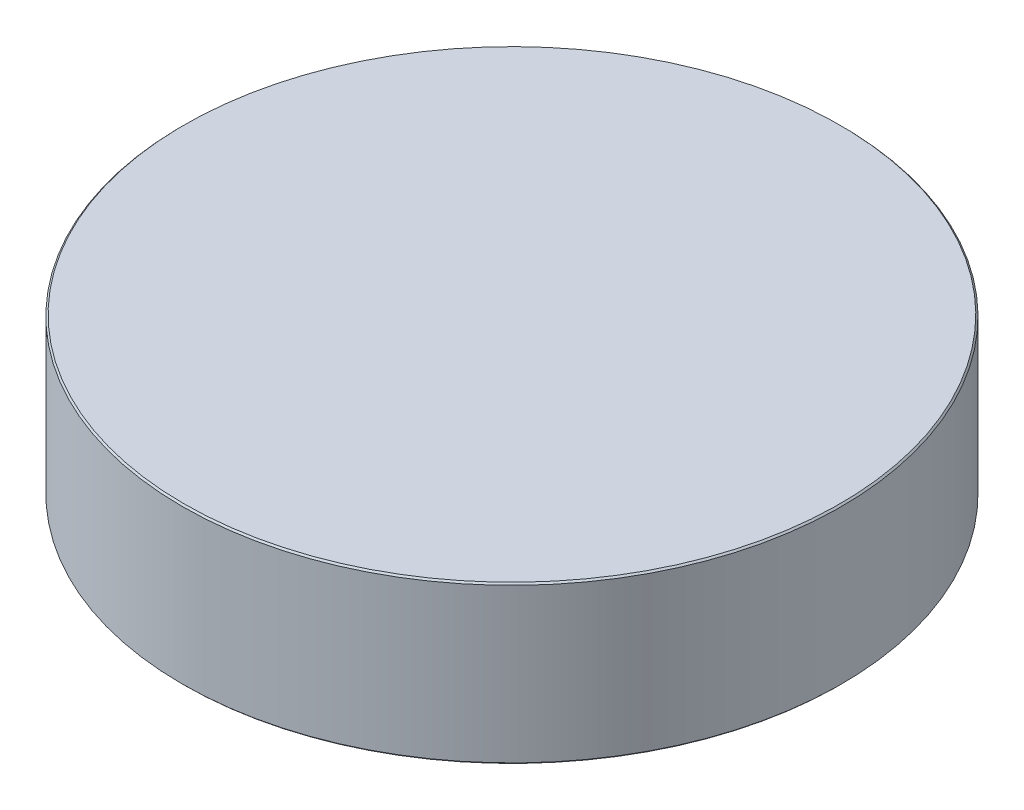
from build123d import *

# Parameters (mm, degrees)
SKETCH_1_R               = 210
SKETCH_1_R_2             = 95.82
EXTRUDE_1_DEPTH          = 100
SKETCH_5_R               = 150
EXTRUDE_4_DEPTH          = 30
PATTERN_CIRCULAR_1_COUNT = 8
CHAMFER_1_SIZE           = 1


with BuildPart() as part:
    # 草图1 → 凸台-拉伸1 (new body)
    with BuildSketch(Plane(origin=(0, 0, 0), x_dir=(1, 0, 0), z_dir=(0, 1, 0))):
        with Locations(Location((0, 0, 0), (0, 0, 270))):
            Circle(SKETCH_1_R)
        with Locations(Location((0, 0, 0), (0, 0, 270))):
            Circle(SKETCH_1_R_2, mode=Mode.SUBTRACT)
    extrude(amount=EXTRUDE_1_DEPTH)

    # 草图5 → 凸台-拉伸4 (add)
    with BuildSketch(Plane(origin=(0, 100, 0), x_dir=(1, 0, 0), z_dir=(0, 1, 0))):
        Circle(SKETCH_5_R)
    extrude(amount=-EXTRUDE_4_DEPTH)

    # 草图8 → M10 螺纹孔1 (revolve, cut)
    with BuildSketch(Plane(origin=(185, 0, 0), x_dir=(0, 0, -1), z_dir=(1, 0, 0))):
        Polygon((0, 0), (0, 30.053657631), (4.25, 27.5), (4.25, 0.775), (5.025, 0), align=None)
    hole_wizard_m10_1 = revolve(axis=Axis((185, -6.35, 0), (0, 1, 0)), mode=Mode.SUBTRACT)

    # 阵列(圆周)1: M10 螺纹孔1 ×8 about axis
    pattern_circular_1_axis = Axis((0, 0, 0), (0, 1, 0))
    for i in range(1, PATTERN_CIRCULAR_1_COUNT):
        add(hole_wizard_m10_1.rotate(pattern_circular_1_axis, i * 360 / PATTERN_CIRCULAR_1_COUNT), mode=Mode.SUBTRACT)

    # 倒角1
    chamfer_1_edges = [part.edges().sort_by_distance(p)[0] for p in [
        (0, 0, -210),
        (0, 100, -210),
        (0, 0, -95.82),
    ]]
    chamfer(chamfer_1_edges, length=CHAMFER_1_SIZE)


solid = part.part
